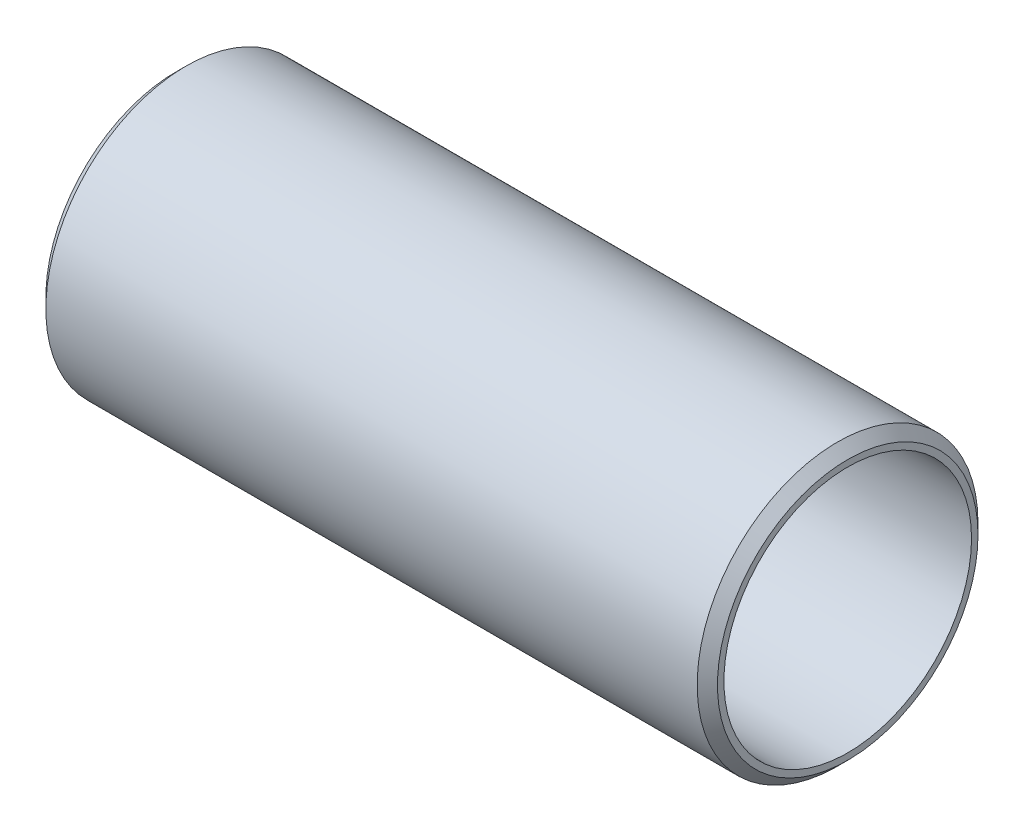
from build123d import *

# Parameters (mm, degrees)
SKETCH1_R                      = 38.05
SKETCH1_R_2                    = 33.55
GB_T3091_2008_76_1X4_5_1_DEPTH = 182
CHAMFER_1_SIZE                 = 2.75


with BuildPart() as part:
    # Sketch1 → 焊接钢管gb∕t3091-2008 Φ76.1X4.5(1) (new body)
    with BuildSketch(Plane.YZ):
        Circle(SKETCH1_R)
        Circle(SKETCH1_R_2, mode=Mode.SUBTRACT)
    extrude(amount=GB_T3091_2008_76_1X4_5_1_DEPTH)

    # 倒角1
    chamfer_1_edges = [part.edges().sort_by_distance(p)[0] for p in [
        (182, -38.05, 0),
        (0, -38.05, 0),
    ]]
    chamfer(chamfer_1_edges, length=CHAMFER_1_SIZE)


solid = part.part
